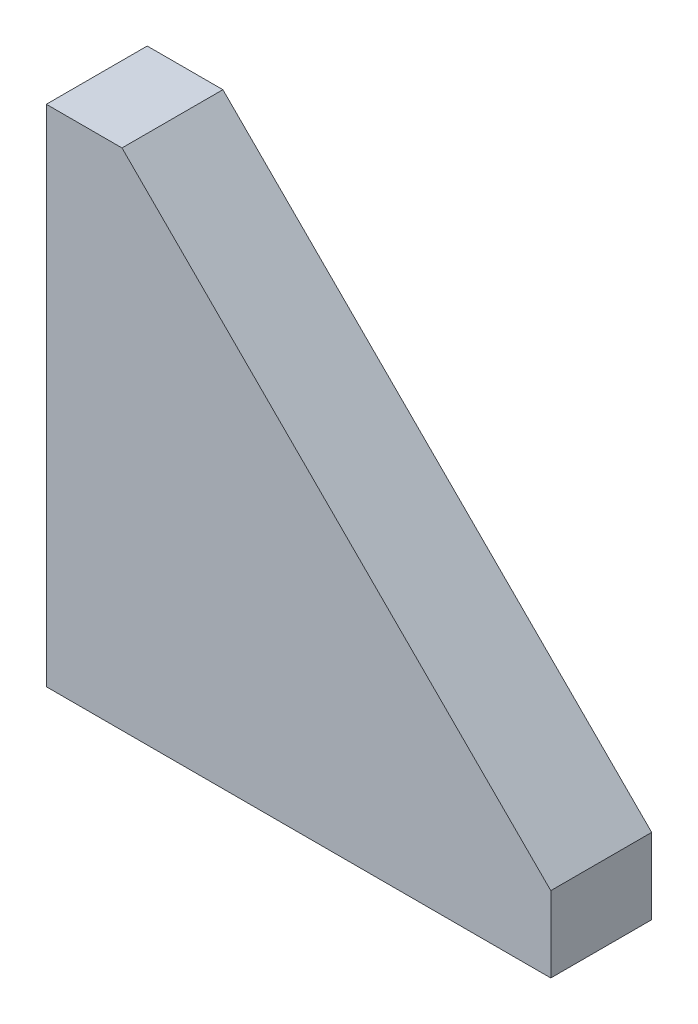
SolidWorks part; units mm, degrees
material "Q235B"
ref_plane "Front Plane" through (0, 0, 0) normal (0, 0, 1) x (1, 0, 0)
ref_plane "Top Plane" through (0, 0, 0) normal (0, 1, 0) x (1, 0, 0)
ref_plane "Right Plane" through (0, 0, 0) normal (1, 0, 0) x (0, 0, -1)
sketch "Sketch1" plane through (0, 0, 0) normal (0, 0, 1) x (1, 0, 0)
  line L0 (0, 0) -> (0, 100)
  line L1 (0, 100) -> (15, 100)
  line L2 (15, 100) -> (100, 15)
  line L3 (100, 15) -> (100, 0)
  line L4 (100, 0) -> (0, 0)
  dimension "D1" = 100
  dimension "D2" = 100
  dimension "D3" = 15
  dimension "D4" = 15
extrude "Boss-Extrude1" add sketch "Sketch1" along normal blind 20
